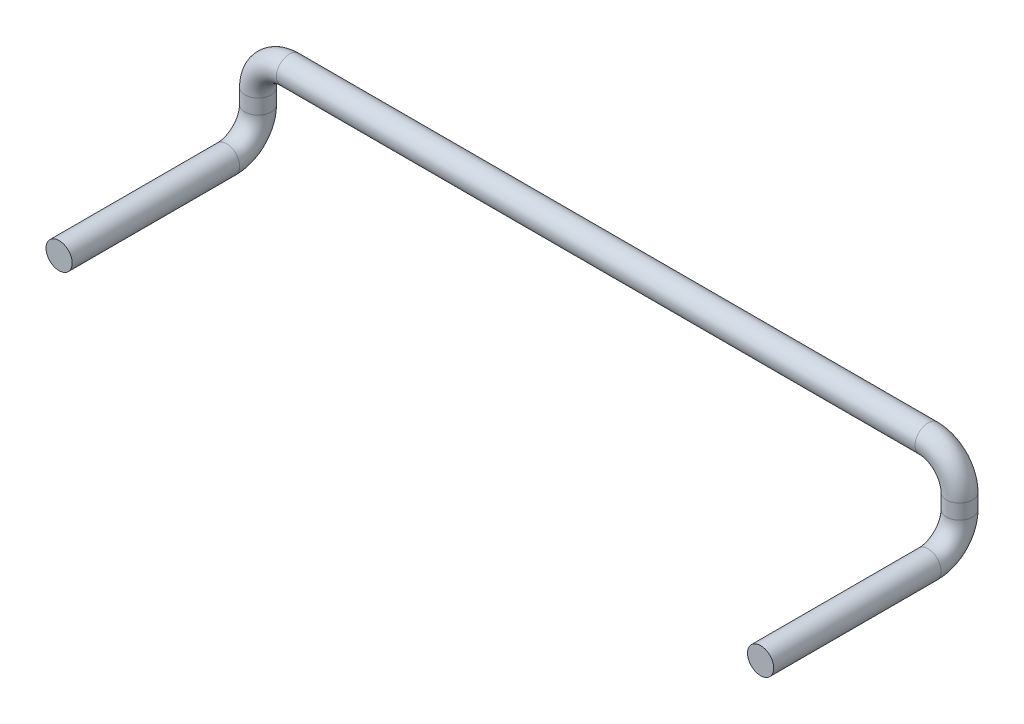
SolidWorks part; units mm, degrees
material "Q235A"
ref_plane "Front Plane" through (0, 0, 0) normal (0, 0, 1) x (1, 0, 0)
ref_plane "Top Plane" through (0, 0, 0) normal (0, 1, 0) x (1, 0, 0)
ref_plane "Right Plane" through (0, 0, 0) normal (1, 0, 0) x (0, 0, -1)
sketch3d "3DSketch2"
  line L0 (-305, 0, 0) -> (305, 0, 0)
  line L1 (-335, -30, 0) -> (-335, -44.162, 0)
  line L2 (335, -30, 0) -> (335, -44.162, 0)
  line L3 (335, -74.162, 30) -> (335, -74.162, 190)
  line L4 (-335, -74.162, 30) -> (-335, -74.162, 190)
  arc A0 (335, -74.162, 30) -> (335, -44.162, 0) centre (335, -44.162, 30) ccw
  arc A1 (-335, -74.162, 30) -> (-335, -44.162, 0) centre (-335, -44.162, 30) ccw
  arc A2 (335, -30, 0) -> (305, 0, 0) centre (305, -30, 0) ccw
  arc A3 (-305, 0, 0) -> (-335, -30, 0) centre (-305, -30, 0) ccw
  point P9 (335, -74.162, 0)
  point P10 (365, -44.162, 30)
  point P13 (-335, -74.162, 0)
  point P14 (-305, -44.162, 30)
  point P17 (335, 0, 0)
  point P18 (305, -30, 30)
  point P21 (-335, 0, 0)
  point P22 (-305, -30, 30)
  dimension "D1" = 30
  dimension "D2" = 30
  dimension "D3" = 30
  dimension "D4" = 670
  dimension "D5" = 190
  dimension "D6" = 80
sweep "Sweep1" add path "3DSketch2" circular profile diameter 25 parameters "D3"=25
